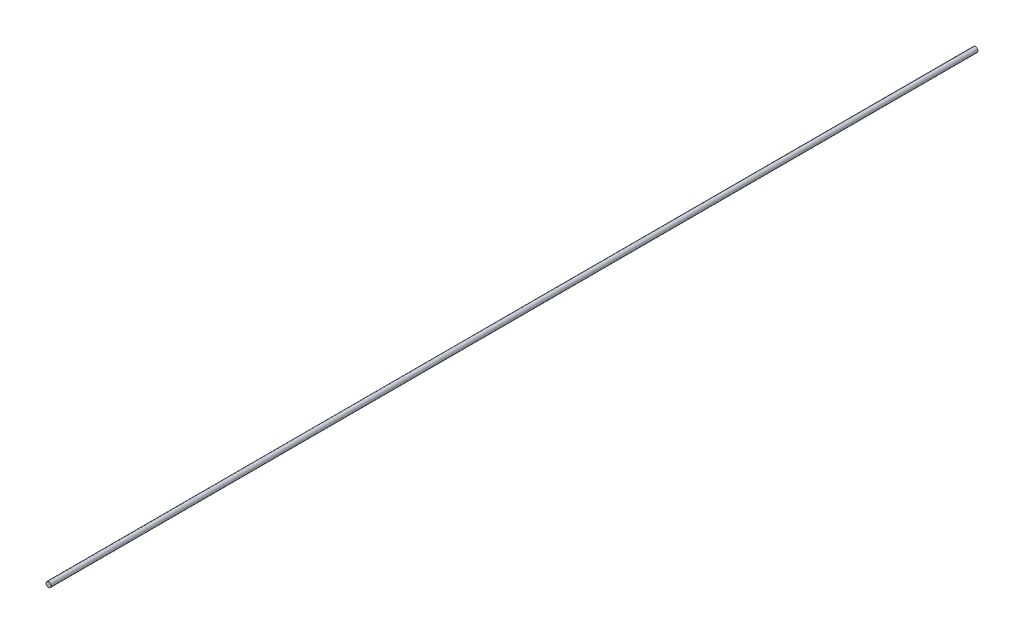
from build123d import *

# Parameters (mm, degrees)
SKETCH1_R           = 15
BOSS_EXTRUDE1_DEPTH = 5500


with BuildPart() as part:
    # Sketch1 → Boss-Extrude1 (new body)
    with BuildSketch(Plane.XY):
        Circle(SKETCH1_R)
    extrude(amount=BOSS_EXTRUDE1_DEPTH)


solid = part.part
